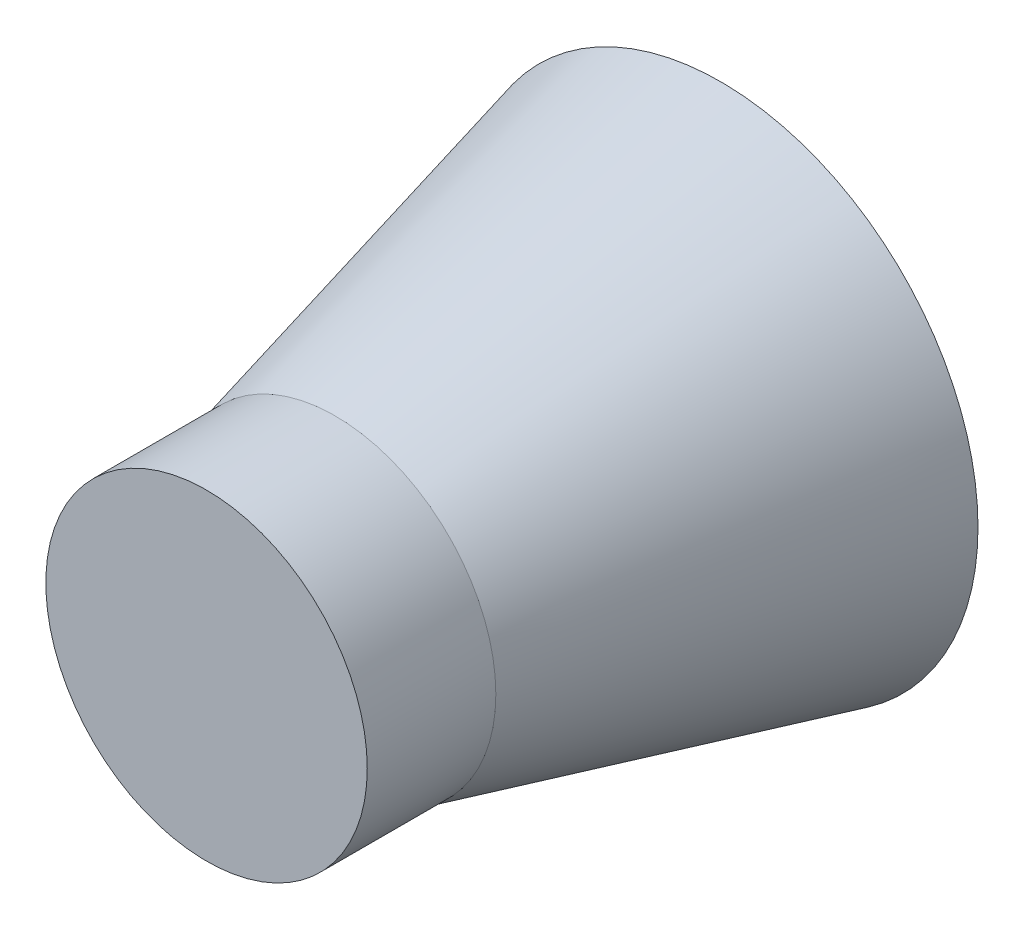
from build123d import *

# Parameters (mm, degrees)
SKETCH2_R           = 12.5
SKETCH1_R           = 20
SKETCH3_R           = 12.5
BOSS_EXTRUDE1_DEPTH = 10


with BuildPart() as part:
    # Sketch2 → Loft1 section 0
    with BuildSketch(Plane(origin=(0, 0, 30), x_dir=(-1, 0, 0), z_dir=(0, 0, -1))):
        Circle(SKETCH2_R)
    # Sketch1 → Loft1 section 1
    with BuildSketch(Plane.XY):
        Circle(SKETCH1_R)
    loft()

    # Sketch3 → Boss-Extrude1 (add)
    with BuildSketch(Plane.XY.offset(30)):
        Circle(SKETCH3_R)
    extrude(amount=BOSS_EXTRUDE1_DEPTH)


solid = part.part
